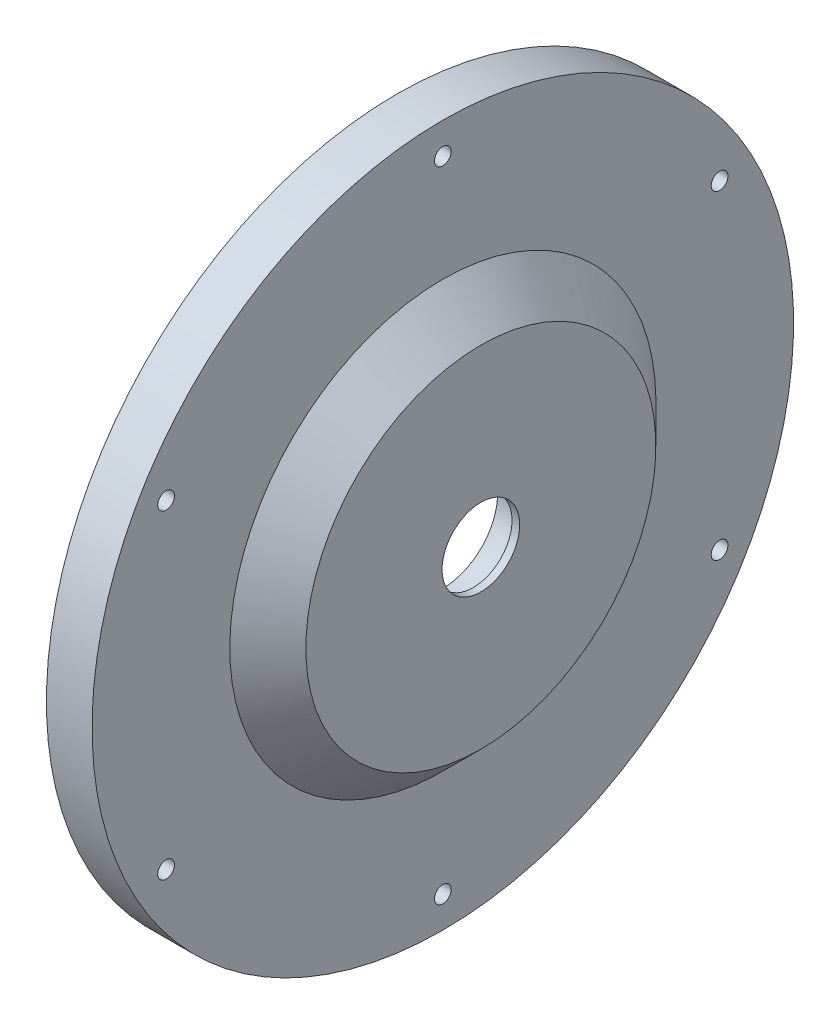
SolidWorks part; units mm, degrees
ref_plane "Front Plane" through (0, 0, 0) normal (0, 0, 1) x (1, 0, 0)
ref_plane "Top Plane" through (0, 0, 0) normal (0, 1, 0) x (1, 0, 0)
ref_plane "Right Plane" through (0, 0, 0) normal (1, 0, 0) x (0, 0, -1)
other "Configuration Table"
sketch "Sketch1" plane through (0, 0, 0) normal (0, 0, 1) x (1, 0, 0)
  line L0 (5, 0) -> (-357.3463, 0) construction
  line L1 (-25, 230.5) -> (-25, 140)
  line L2 (0, 115) -> (0, 25.5)
  line L3 (-55, 230.5) -> (-55, 215.5)
  line L4 (-55, 205.5) -> (-55, 82.5)
  line L5 (-25, 230.5) -> (-55, 230.5)
  line L6 (-55, 82.5) -> (-25, 52.5)
  line L7 (-25, 36) -> (-25, 52.5)
  line L8 (-25, 140) -> (0, 115)
  line L10 (-55, 215.5) -> (-55, 205.5)
  line L13 (5, 0) -> (-357.3463, 0) construction
  line L14 (-6, 36) -> (-25, 36)
  line L15 (-5, 35) -> (-5, 25.5)
  line L16 (-5, 25.5) -> (0, 25.5)
  arc A0 (-5, 35) -> (-6, 36) centre (-6, 35) ccw
revolve "Revolve1" add sketch "Sketch1" angle 360 about L0
sketch "Sketch2" plane through (-55, 0, 0) normal (-1, 0, 0) x (0, 0, 1)
  circle A0 centre (0, 210) radius 5.5
  circle A1 centre (181.8653, 105) radius 5.5
  circle A2 centre (181.8653, -105) radius 5.5
  circle A3 centre (0, -210) radius 5.5
  circle A4 centre (-181.8653, -105) radius 5.5
  circle A5 centre (-181.8653, 105) radius 5.5
  point P15 (0, 0)
  dimension "D1" = 6
extrude "Cut-Extrude1" cut sketch "Sketch2" against normal blind 85
